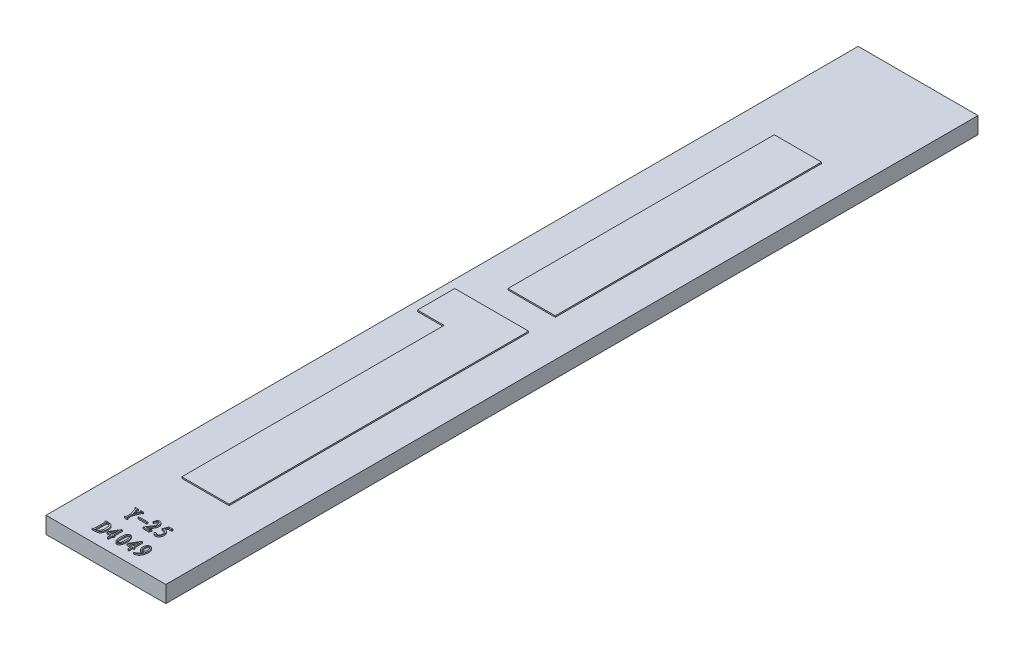
from build123d import *

# Parameters (mm, degrees)
SKETCH1_W           = 9
SKETCH1_H           = 61
BOSS_EXTRUDE1_DEPTH = 1.25
SKETCH2_W           = 3.55
SKETCH2_H           = 20
BOSS_EXTRUDE2_DEPTH = 0.1
SKETCH4_W           = 0.666666667
SKETCH4_H           = 0.083333333
BOSS_EXTRUDE3_DEPTH = 0.1
BOSS_EXTRUDE4_DEPTH = 0.1


with BuildPart() as part:
    # Sketch1 → Boss-Extrude1 (new body)
    with BuildSketch(Plane(origin=(0, 0, 0), x_dir=(1, 0, 0), z_dir=(0, 1, 0))):
        with Locations((4.5, 30.5)):
            Rectangle(SKETCH1_W, SKETCH1_H)
    extrude(amount=BOSS_EXTRUDE1_DEPTH)

    # Sketch2 → Boss-Extrude2 (add)
    with BuildSketch(Plane(origin=(0, 1.25, 0), x_dir=(1, 0, 0), z_dir=(0, 1, 0))):
        Polygon((2.7, 7.5), (6.25, 7.5), (6.25, 30), (0.7, 30), (0.7, 27.2), (2.7, 27.2), align=None)
        with Locations((4.475, 42)):
            Rectangle(SKETCH2_W, SKETCH2_H)
    extrude(amount=BOSS_EXTRUDE2_DEPTH)

    # Sketch4 → Boss-Extrude3 (add)
    with BuildSketch(Plane(origin=(0, 1.25, 0), x_dir=(1, 0, 0), z_dir=(0, 1, 0))):
        with BuildLine():
            add(Edge.make_bspline(
                [(3.112430638, 2.801603821), (3.117581172, 2.801718451), (3.127409954, 2.801937201), (3.141398685, 2.803908272), (3.153687941, 2.807150558), (3.164467449, 2.811513751), (3.173308112, 2.817610015), (3.180890686, 2.824709906), (3.186470888, 2.833463912), (3.188691334, 2.839981993), (3.18981159, 2.843270488)],
                knots=[0, 0, 0, 0, 1.302072691, 2.484749895, 3.562139971, 4.511379366, 5.408236895, 6.262493732, 7.123395447, 8, 8, 8, 8], degree=3))
            Line((3.18981159, 2.843270488), (3.18981159, 3.188508583))
            Line((3.18981159, 3.188508583), (3.041002066, 3.652794297))
            add(Edge.make_bspline(
                [(3.041002066, 3.652794297), (3.038871047, 3.658879382), (3.034760977, 3.670615605), (3.026438221, 3.686643453), (3.016164612, 3.700185527), (3.004024748, 3.711065386), (2.990457739, 3.719976466), (2.974917219, 3.725734702), (2.957946602, 3.729752217), (2.946010572, 3.730030647), (2.93981159, 3.730175249)],
                knots=[0, 0, 0, 0, 1.120090753, 2.160304349, 3.126304926, 4.057980278, 4.983061327, 5.929772381, 6.924826447, 8, 8, 8, 8], degree=3))
            Line((2.93981159, 3.730175249), (2.93981159, 3.765889535))
            Line((2.93981159, 3.765889535), (3.18981159, 3.765889535))
            Line((3.18981159, 3.765889535), (3.18981159, 3.730175249))
            add(Edge.make_bspline(
                [(3.18981159, 3.730175249), (3.185235193, 3.729984155), (3.176767714, 3.729630583), (3.165196849, 3.726598153), (3.155932393, 3.721482658), (3.149071491, 3.71401788), (3.14520736, 3.704272832), (3.143441674, 3.692750595), (3.144607976, 3.679220776), (3.146899509, 3.669812381), (3.148144923, 3.664699059)],
                knots=[0, 0, 0, 0, 1.148008426, 2.124103102, 2.975698962, 3.77274816, 4.616104197, 5.568887894, 6.67872674, 8, 8, 8, 8], degree=3))
            Line((3.148144923, 3.664699059), (3.261240161, 3.265889535))
            Line((3.261240161, 3.265889535), (3.416002066, 3.664699059))
            add(Edge.make_bspline(
                [(3.416002066, 3.664699059), (3.417241452, 3.669807437), (3.419522538, 3.679209394), (3.419720463, 3.692904094), (3.416629771, 3.70462606), (3.410469082, 3.714374984), (3.401020003, 3.721691407), (3.388689171, 3.726643043), (3.3735186, 3.729617596), (3.362445838, 3.729979958), (3.356478257, 3.730175249)],
                knots=[0, 0, 0, 0, 1.154411579, 2.124691882, 2.979940139, 3.787374271, 4.615750981, 5.564913494, 6.687628387, 8, 8, 8, 8], degree=3))
            Line((3.356478257, 3.730175249), (3.356478257, 3.765889535))
            Line((3.356478257, 3.765889535), (3.570763971, 3.765889535))
            Line((3.570763971, 3.765889535), (3.570763971, 3.730175249))
            add(Edge.make_bspline(
                [(3.570763971, 3.730175249), (3.565097471, 3.730076594), (3.554231253, 3.729887411), (3.538765239, 3.727687608), (3.524922451, 3.724040734), (3.512874507, 3.71863394), (3.502273069, 3.712087558), (3.493551288, 3.703683739), (3.486264134, 3.693911629), (3.483092248, 3.68638571), (3.481478257, 3.682556202)],
                knots=[0, 0, 0, 0, 1.254413916, 2.405494607, 3.452028913, 4.413990841, 5.321667416, 6.196791605, 7.082450772, 8, 8, 8, 8], degree=3))
            Line((3.481478257, 3.682556202), (3.279097304, 3.188508583))
            Line((3.279097304, 3.188508583), (3.279097304, 2.849222868))
            add(Edge.make_bspline(
                [(3.279097304, 2.849222868), (3.280249643, 2.845399393), (3.282472632, 2.838023482), (3.288614447, 2.828300632), (3.296038715, 2.819575939), (3.306095356, 2.813201128), (3.317462547, 2.807606634), (3.330936829, 2.804466218), (3.346008769, 2.801758023), (3.356756025, 2.801657106), (3.362430638, 2.801603821)],
                knots=[0, 0, 0, 0, 0.914764513, 1.764682586, 2.627130839, 3.527870916, 4.481226645, 5.531530322, 6.696633754, 8, 8, 8, 8], degree=3))
            Line((3.362430638, 2.801603821), (3.362430638, 2.765889535))
            Line((3.362430638, 2.765889535), (3.112430638, 2.765889535))
            Line((3.112430638, 2.765889535), (3.112430638, 2.801603821))
        make_face()
        with Locations((4.023144924, 3.248032392)):
            Rectangle(SKETCH4_W, SKETCH4_H)
        with BuildLine():
            Line((4.654097304, 2.86112763), (4.886240161, 2.86112763))
            add(Edge.make_bspline(
                [(4.886240161, 2.86112763), (4.89120182, 2.86232734), (4.90117029, 2.864737676), (4.915560668, 2.870641239), (4.929700036, 2.878182253), (4.943174184, 2.887916069), (4.956389045, 2.899410907), (4.969325445, 2.912511555), (4.981761976, 2.927712183), (4.989418066, 2.938746492), (4.993383019, 2.944460964)],
                knots=[0, 0, 0, 0, 0.878382117, 1.764757949, 2.67116336, 3.633749211, 4.621162033, 5.686586957, 6.801924741, 8, 8, 8, 8], degree=3))
            Line((4.993383019, 2.944460964), (5.029097304, 2.944460964))
            Line((5.029097304, 2.944460964), (4.969573495, 2.765889535))
            Line((4.969573495, 2.765889535), (4.523144923, 2.765889535))
            Line((4.523144923, 2.765889535), (4.523144923, 2.801603821))
            add(Edge.make_bspline(
                [(4.523144923, 2.801603821), (4.533276428, 2.815720099), (4.55307626, 2.843307307), (4.582191934, 2.883534346), (4.609687964, 2.921982472), (4.635203081, 2.958826199), (4.659995164, 2.993331759), (4.682457882, 3.026525689), (4.703962794, 3.057427651), (4.723540269, 3.086730851), (4.741958777, 3.113892248), (4.758339318, 3.139589289), (4.773698078, 3.163111499), (4.787252557, 3.184935829), (4.799551189, 3.204707669), (4.809768296, 3.222884641), (4.818954916, 3.238931677), (4.833272238, 3.266385123), (4.850738573, 3.306191809), (4.867619022, 3.359471501), (4.878179555, 3.412423136), (4.881036118, 3.464353914), (4.879376769, 3.513489546), (4.873684879, 3.558578481), (4.864697368, 3.598895473), (4.853764424, 3.629098408), (4.842943811, 3.650303598), (4.83309138, 3.663744769), (4.821745626, 3.675055001), (4.80906807, 3.684545272), (4.794681549, 3.691604059), (4.778861246, 3.696685782), (4.761580121, 3.699702913), (4.743316465, 3.700720903), (4.724975364, 3.699932686), (4.707450291, 3.697051569), (4.691225574, 3.692436175), (4.676254184, 3.686043249), (4.662629825, 3.677584194), (4.650483442, 3.667013355), (4.639321173, 3.654944269), (4.626791499, 3.635935642), (4.613390541, 3.610003395), (4.599782154, 3.576770948), (4.589437113, 3.541196018), (4.584949623, 3.516524665), (4.582668733, 3.503984773)],
                knots=[0, 0, 0, 0, 1.69631524, 3.315080701, 4.847930107, 6.310785452, 7.69019844, 8.995595461, 10.223400104, 11.365530615, 12.436016475, 13.427008482, 14.340408662, 15.178432467, 15.935125256, 16.613185454, 17.213845292, 17.740106165, 19.635490543, 21.448390511, 23.187434146, 24.891106341, 26.513476491, 27.981722556, 29.321731269, 30.538418994, 31.106445655, 31.640232205, 32.157665963, 32.665613008, 33.178952369, 33.714375566, 34.282900357, 34.88659439, 35.497070761, 36.071449824, 36.616400871, 37.140161911, 37.655752223, 38.174775033, 38.708031004, 39.255244051, 40.391297374, 41.552997966, 42.756244035, 44, 44, 44, 44], degree=3))
            Line((4.582668733, 3.503984773), (4.546954447, 3.503984773))
            add(Edge.make_bspline(
                [(4.546954447, 3.503984773), (4.548447235, 3.517302462), (4.551300798, 3.542760099), (4.557339962, 3.579000045), (4.56404142, 3.611619097), (4.571712465, 3.640641723), (4.580246877, 3.66608972), (4.589560754, 3.688066149), (4.600036933, 3.706396295), (4.61535225, 3.725273796), (4.635882965, 3.743774302), (4.661279663, 3.76208135), (4.68838557, 3.774330269), (4.716372054, 3.781352569), (4.744491904, 3.784117904), (4.772334047, 3.785855753), (4.799755235, 3.784190721), (4.822382831, 3.781726559), (4.840496661, 3.777921838), (4.853888586, 3.772428175), (4.867323438, 3.765252243), (4.880767208, 3.756167143), (4.894225861, 3.745052633), (4.907614233, 3.732053567), (4.920946192, 3.717040435), (4.934253689, 3.700336944), (4.946982488, 3.681691422), (4.957644837, 3.66079171), (4.966993301, 3.638269936), (4.97441095, 3.613800999), (4.980392081, 3.58751437), (4.98451604, 3.559280674), (4.986808626, 3.529232083), (4.987805221, 3.497662748), (4.986555747, 3.464929179), (4.982450655, 3.431573766), (4.976115453, 3.397807784), (4.966974891, 3.363619089), (4.955064583, 3.329192403), (4.940503965, 3.29439891), (4.923930706, 3.259042026), (4.903862761, 3.223445528), (4.881547087, 3.186248104), (4.856694052, 3.146974312), (4.829185585, 3.10526936), (4.799591103, 3.060883918), (4.766827012, 3.014428311), (4.731462609, 2.965530295), (4.693935471, 2.913905961), (4.667600681, 2.879017151), (4.654097304, 2.86112763)],
                knots=[0, 0, 0, 0, 1.250310692, 2.390051031, 3.426959399, 4.356778373, 5.189484751, 5.929631335, 6.581185539, 7.151993547, 8.190374716, 9.151012377, 10.062443573, 10.947251191, 11.830995274, 12.695997373, 13.547300594, 14.390193962, 14.819366142, 15.268874171, 15.735172317, 16.239174092, 16.780034109, 17.361978296, 17.978718407, 18.652343773, 19.354140052, 20.08104892, 20.837471312, 21.626987473, 22.463749812, 23.351104713, 24.286746534, 25.274582321, 26.297151914, 27.339939007, 28.40778998, 29.500603315, 30.639105254, 31.804326119, 33.018982859, 34.280469881, 35.615254974, 37.066839227, 38.616913391, 40.277264392, 42.044606227, 43.921109359, 45.908515667, 48, 48, 48, 48], degree=3))
        make_face()
        with BuildLine():
            add(Edge.make_bspline(
                [(5.701716352, 3.075413345), (5.701486986, 3.085642364), (5.701036134, 3.105749033), (5.696742862, 3.13523725), (5.689651408, 3.163356716), (5.679957419, 3.190233341), (5.667316498, 3.215755997), (5.651673853, 3.239854551), (5.633634006, 3.262913658), (5.612557201, 3.284340213), (5.588580744, 3.304151292), (5.561384932, 3.321788448), (5.530874395, 3.337012951), (5.497255551, 3.34994495), (5.460520739, 3.36068329), (5.420745897, 3.369271613), (5.377777295, 3.375357704), (5.348043177, 3.377748552), (5.332668733, 3.378984773)],
                knots=[0, 0, 0, 0, 0.917758673, 1.803991995, 2.667923906, 3.517226481, 4.363886405, 5.218398847, 6.092022264, 6.987632944, 7.910780789, 8.878660533, 9.890520551, 10.966063617, 12.107781048, 13.322690178, 14.615659297, 16, 16, 16, 16], degree=3))
            Line((5.332668733, 3.378984773), (5.487430638, 3.765889535))
            Line((5.487430638, 3.765889535), (5.785049685, 3.765889535))
            Line((5.785049685, 3.765889535), (5.743383019, 3.67065144))
            Line((5.743383019, 3.67065144), (5.499335399, 3.67065144))
            Line((5.499335399, 3.67065144), (5.421954447, 3.474222868))
            add(Edge.make_bspline(
                [(5.421954447, 3.474222868), (5.43543744, 3.4716654), (5.461759706, 3.466672563), (5.499713892, 3.45665811), (5.535158843, 3.44519123), (5.568293007, 3.432638487), (5.598509706, 3.417586893), (5.626610132, 3.401687165), (5.65216044, 3.384009142), (5.675058682, 3.364442925), (5.695678968, 3.34295099), (5.713348894, 3.318771687), (5.728278946, 3.291962691), (5.740300071, 3.262537324), (5.749783179, 3.23055874), (5.756614191, 3.196026166), (5.760422137, 3.158838789), (5.761664612, 3.119872591), (5.760405692, 3.080613578), (5.756540175, 3.04248845), (5.749730248, 3.00635462), (5.740207208, 2.972132075), (5.728099765, 2.939861114), (5.713317374, 2.909441514), (5.695589482, 2.881112397), (5.675333627, 2.855114525), (5.653707148, 2.831470576), (5.631118096, 2.810521813), (5.607717977, 2.792701367), (5.583858742, 2.777489241), (5.559239852, 2.765473359), (5.533912363, 2.756627208), (5.50796705, 2.750602231), (5.481844605, 2.747663712), (5.456572353, 2.747108423), (5.433109887, 2.746893086), (5.411849266, 2.748058321), (5.392831828, 2.749903305), (5.375992566, 2.752919751), (5.361440855, 2.757055092), (5.348984611, 2.762079917), (5.335834668, 2.77014126), (5.323067621, 2.781853056), (5.31148258, 2.797201293), (5.304299812, 2.813847059), (5.302347152, 2.831115572), (5.303741859, 2.847567865), (5.309751869, 2.86205242), (5.31929329, 2.874098869), (5.332602466, 2.882409886), (5.34718887, 2.887872427), (5.362403718, 2.890980111), (5.377603387, 2.889498356), (5.392882429, 2.885541508), (5.407769225, 2.876192595), (5.420403414, 2.860443262), (5.431421013, 2.839088668), (5.436837211, 2.822576479), (5.43981159, 2.813508583)],
                knots=[0, 0, 0, 0, 1.545808417, 3.017815207, 4.418618593, 5.742433702, 7.0051059, 8.217933456, 9.377803328, 10.499454895, 11.606341578, 12.725790828, 13.863703459, 15.05531972, 16.299589297, 17.616447294, 19.01536536, 20.506504195, 22.005917965, 23.437769934, 24.819653994, 26.143469103, 27.435204746, 28.697876944, 29.947616226, 31.192987171, 32.406012533, 33.554448986, 34.658979797, 35.715647213, 36.737654915, 37.737934401, 38.732095913, 39.732375399, 40.693368948, 41.57927611, 42.375186034, 43.091112019, 43.730941629, 44.299581586, 44.793167942, 45.239032996, 46.030451586, 46.729273299, 47.393545671, 48.044632898, 48.66911846, 49.233401885, 49.786829744, 50.372396319, 50.975153468, 51.538707531, 52.103233868, 52.679834753, 53.304704394, 54.044690326, 54.926214758, 56, 56, 56, 56], degree=3))
            add(Edge.make_bspline(
                [(5.43981159, 2.813508583), (5.452162474, 2.813730705), (5.475876657, 2.81415719), (5.509958499, 2.817086894), (5.540846431, 2.822590547), (5.568625154, 2.83002199), (5.593348612, 2.839418352), (5.614965526, 2.851061509), (5.633396893, 2.865093814), (5.648569184, 2.881530779), (5.661154426, 2.899888817), (5.671895492, 2.919845687), (5.681329596, 2.941387369), (5.688659521, 2.964862791), (5.694671528, 2.990039069), (5.698768945, 3.016953386), (5.701196569, 3.045606431), (5.701539422, 3.065267281), (5.701716352, 3.075413345)],
                knots=[0, 0, 0, 0, 1.375740717, 2.641476338, 3.805546928, 4.86588406, 5.840245249, 6.745008832, 7.591426724, 8.40803176, 9.225456845, 10.064241315, 10.929448168, 11.840631474, 12.799571018, 13.81021633, 14.869953018, 16, 16, 16, 16], degree=3))
        make_face()
    extrude(amount=BOSS_EXTRUDE3_DEPTH)

    # Sketch6 → Boss-Extrude4 (add)
    # profile 1 of 5: a face of its own
    with BuildSketch(Plane(origin=(0, 1.25, 0), x_dir=(1, 0, 0), z_dir=(0, 1, 0))):
        with BuildLine():
            add(Edge.make_bspline(
                [(4.739090128, 1.653953152), (4.74464243, 1.642572568), (4.756080648, 1.619127585), (4.770090567, 1.581179998), (4.78173022, 1.539900287), (4.792129577, 1.495458742), (4.799462129, 1.447517107), (4.805590908, 1.396286512), (4.809112201, 1.341684335), (4.810898493, 1.284845406), (4.81045001, 1.227851981), (4.807984239, 1.172740122), (4.802820651, 1.120595486), (4.79583916, 1.071352755), (4.785694739, 1.025207725), (4.774035272, 0.981871076), (4.759669722, 0.941540599), (4.743002768, 0.904504254), (4.724779757, 0.87097452), (4.704543999, 0.84189206), (4.68329615, 0.816917232), (4.66035724, 0.796602988), (4.636132366, 0.780517889), (4.610151148, 0.769502524), (4.582891587, 0.76239714), (4.554637982, 0.760433152), (4.526466096, 0.762410127), (4.499520979, 0.769409596), (4.474056632, 0.780613047), (4.450346131, 0.796493115), (4.428273135, 0.816931528), (4.408103659, 0.84189232), (4.389229563, 0.871061402), (4.37230918, 0.90455865), (4.356981203, 0.941628627), (4.343804115, 0.981976788), (4.332651247, 1.025214813), (4.323343113, 1.071416812), (4.316451231, 1.120604874), (4.311388021, 1.172754414), (4.30839382, 1.227842539), (4.307273485, 1.284832076), (4.308390658, 1.341674761), (4.311369639, 1.396250759), (4.31642398, 1.447521946), (4.323295771, 1.495397308), (4.332621016, 1.539913354), (4.343741557, 1.581111797), (4.356853888, 1.619088649), (4.372384042, 1.653289996), (4.388671741, 1.68395939), (4.404766472, 1.711192807), (4.420448299, 1.73484588), (4.436199733, 1.754716472), (4.451672302, 1.770895068), (4.467111883, 1.783348183), (4.482350471, 1.792335746), (4.502597497, 1.798509563), (4.527483962, 1.80145812), (4.556772324, 1.803406045), (4.585692197, 1.801481322), (4.609794539, 1.798536637), (4.62928061, 1.792270512), (4.644037918, 1.783268711), (4.659244462, 1.770901183), (4.674463223, 1.754575766), (4.69048871, 1.734888233), (4.706319027, 1.711133372), (4.722967082, 1.683975146), (4.733533603, 1.664299707), (4.739090128, 1.653953152)],
                knots=[0, 0, 0, 0, 1.017482002, 2.096100383, 3.245942481, 4.464050679, 5.762547996, 7.14234081, 8.61084165, 10.159330965, 11.713051354, 13.191629558, 14.592407491, 15.924128784, 17.187093352, 18.388106522, 19.529785616, 20.624461962, 21.650397864, 22.59267832, 23.467967375, 24.27990102, 25.04837719, 25.794596655, 26.538216003, 27.302571261, 28.061036816, 28.798932034, 29.528910178, 30.287513756, 31.081892824, 31.938135587, 32.860653577, 33.869922099, 34.950544627, 36.082630963, 37.279058791, 38.538412174, 39.86928151, 41.270059442, 42.749251193, 44.303207409, 45.851257185, 47.318652545, 48.695913765, 49.991707208, 51.204762542, 52.349814403, 53.420378675, 54.430476733, 55.365954973, 56.210914966, 56.97280072, 57.645375484, 58.246956243, 58.768225076, 59.23644892, 59.658660367, 60.459035494, 61.245821967, 62.014910966, 62.786084466, 63.191470614, 63.649445639, 64.166108078, 64.763585019, 65.439859612, 66.205059072, 67.056109835, 68, 68, 68, 68], degree=3))
        make_face()
        with BuildLine():
            add(Edge.make_bspline(
                [(4.447423462, 0.942533399), (4.45015124, 0.934280177), (4.455324763, 0.918627062), (4.463668268, 0.896733556), (4.472177652, 0.877563103), (4.481242535, 0.86140356), (4.48998097, 0.847586904), (4.499205212, 0.836702417), (4.508672128, 0.8284822), (4.521488613, 0.821796026), (4.537649907, 0.817518961), (4.55676736, 0.815586199), (4.575559593, 0.817448286), (4.590941859, 0.82187829), (4.603106258, 0.828444609), (4.611917226, 0.836881525), (4.620921613, 0.84763415), (4.6296653, 0.861398519), (4.638706078, 0.877603979), (4.64739944, 0.896805283), (4.656502201, 0.918565119), (4.665349639, 0.943480053), (4.673843754, 0.971803888), (4.681019157, 1.004228942), (4.687069994, 1.040812178), (4.692145926, 1.081552026), (4.695674703, 1.126505968), (4.698677318, 1.175523003), (4.699962893, 1.228828077), (4.700794856, 1.284979002), (4.699958194, 1.341350341), (4.698669013, 1.395315946), (4.695644825, 1.445506692), (4.692129825, 1.492074816), (4.687033741, 1.534866975), (4.680908997, 1.573999931), (4.673787359, 1.609430638), (4.665373874, 1.641150116), (4.656167403, 1.669227855), (4.645252263, 1.693458648), (4.633521115, 1.714237559), (4.620231093, 1.731197543), (4.605774493, 1.744659839), (4.589792593, 1.75404882), (4.572655432, 1.760128449), (4.554635709, 1.761595054), (4.53663999, 1.760087108), (4.519639459, 1.754160466), (4.503996798, 1.74455698), (4.489767344, 1.73125626), (4.476960428, 1.714184779), (4.465615058, 1.693483604), (4.455433203, 1.6691759), (4.446863001, 1.641125882), (4.439127606, 1.609403429), (4.432646755, 1.573982974), (4.427238837, 1.534837763), (4.422573592, 1.492057458), (4.419193888, 1.445505575), (4.416510621, 1.395308072), (4.415008597, 1.341352597), (4.414686135, 1.284979036), (4.415004624, 1.228825746), (4.416502474, 1.175531133), (4.419165693, 1.126507154), (4.42256019, 1.081571018), (4.427198612, 1.040841585), (4.432571317, 1.004258772), (4.438997654, 0.971812365), (4.444725668, 0.951908002), (4.447423462, 0.942533399)],
                knots=[0, 0, 0, 0, 0.837318371, 1.588063525, 2.256595512, 2.855528614, 3.371956206, 3.828855314, 4.22588514, 4.571123252, 5.211979743, 5.823459694, 6.413795224, 7.020708911, 7.35352855, 7.734517243, 8.186840906, 8.703268497, 9.302201599, 9.973688479, 10.732303747, 11.574278234, 12.519566182, 13.57927191, 14.771097569, 16.090919092, 17.53312208, 19.114568118, 20.821487341, 22.669402391, 24.524396641, 26.252546021, 27.869331708, 29.367981921, 30.751055998, 32.01973937, 33.183262711, 34.230790244, 35.180046561, 36.02611856, 36.787470794, 37.472993127, 38.094473346, 38.678492207, 39.247161774, 39.830450691, 40.406693806, 40.975363373, 41.547240947, 42.16349736, 42.840337187, 43.594678906, 44.432266602, 45.374926275, 46.417201326, 47.576646698, 48.842185377, 50.223664003, 51.72176228, 53.33816041, 55.06630979, 56.92123649, 58.76908373, 60.476002953, 62.057052771, 63.498682212, 64.816831727, 66.005309347, 67.060535974, 68, 68, 68, 68], degree=3))
        make_face(mode=Mode.SUBTRACT)
    # profile 2 of 5: a face of its own
    with BuildSketch(Plane(origin=(0, 1.25, 0), x_dir=(1, 0, 0), z_dir=(0, 1, 0))):
        with BuildLine():
            add(Edge.make_bspline(
                [(2.682652738, 0.820619819), (2.687814996, 0.820747188), (2.697713443, 0.820991413), (2.711724891, 0.82399898), (2.72428452, 0.828396042), (2.734795525, 0.835311895), (2.744011538, 0.843602336), (2.751205571, 0.854143168), (2.7568441, 0.866448456), (2.758943551, 0.875462889), (2.760033691, 0.880143629)],
                knots=[0, 0, 0, 0, 1.150371848, 2.20579727, 3.187074628, 4.101909412, 4.995909181, 5.938140712, 6.929380532, 8, 8, 8, 8], degree=3))
            Line((2.760033691, 0.880143629), (2.760033691, 1.707524581))
            add(Edge.make_bspline(
                [(2.760033691, 1.707524581), (2.758443004, 1.710812895), (2.755295218, 1.71732009), (2.748894973, 1.726011557), (2.740906138, 1.733141064), (2.731867695, 1.739240833), (2.721235161, 1.743533857), (2.709570085, 1.746856213), (2.69653572, 1.748866561), (2.687436631, 1.749079365), (2.682652738, 1.749191248)],
                knots=[0, 0, 0, 0, 0.935251606, 1.850754977, 2.744090757, 3.668849662, 4.631031247, 5.668626053, 6.774268272, 8, 8, 8, 8], degree=3))
            Line((2.682652738, 1.749191248), (2.682652738, 1.784905533))
            Line((2.682652738, 1.784905533), (2.926700357, 1.784905533))
            add(Edge.make_bspline(
                [(2.926700357, 1.784905533), (2.943042628, 1.783612512), (2.974770561, 1.781102158), (3.020483162, 1.773330759), (3.062951049, 1.762613783), (3.10205121, 1.748568568), (3.137818869, 1.731284485), (3.170337397, 1.711042469), (3.199161528, 1.687111848), (3.225105015, 1.660319453), (3.247463599, 1.629639503), (3.267035621, 1.595459272), (3.283127158, 1.55732135), (3.296747203, 1.515544911), (3.306801943, 1.469881778), (3.314373233, 1.420476471), (3.318542649, 1.367287276), (3.32008505, 1.311434246), (3.318518179, 1.255067595), (3.314293891, 1.200352208), (3.30675905, 1.148452838), (3.29651409, 1.099271684), (3.283026566, 1.052944399), (3.266845926, 1.00925936), (3.247168493, 0.968621529), (3.228890179, 0.936387516), (3.211298577, 0.91236602), (3.194957623, 0.895902888), (3.176155639, 0.880301651), (3.154275438, 0.866357018), (3.13006291, 0.853036488), (3.102932485, 0.841189824), (3.073152227, 0.830481879), (3.040654826, 0.820697374), (3.005318082, 0.812574418), (2.967357917, 0.804891382), (2.926551228, 0.798994262), (2.8830661, 0.793524113), (2.836794797, 0.789746909), (2.787845168, 0.786795769), (2.736158705, 0.785388905), (2.700804369, 0.785069515), (2.682652738, 0.784905533)],
                knots=[0, 0, 0, 0, 1.172240782, 2.275863581, 3.312445736, 4.301874109, 5.242329815, 6.149506285, 7.034618434, 7.915787832, 8.810541892, 9.7429559, 10.727273807, 11.766292461, 12.882167044, 14.068002195, 15.339269347, 16.696047765, 18.063336138, 19.371279044, 20.619512496, 21.812411093, 22.961989922, 24.06825131, 25.140452033, 26.189001953, 26.714691608, 27.264885542, 27.843741229, 28.459045194, 29.117732443, 29.81908992, 30.57407251, 31.380710697, 32.24521049, 33.166893033, 34.150494761, 35.193760284, 36.301756457, 37.470786713, 38.701450783, 40, 40, 40, 40], degree=3))
            Line((2.682652738, 0.784905533), (2.682652738, 0.820619819))
        make_face()
        with BuildLine():
            add(Edge.make_bspline(
                [(2.849319405, 0.862286486), (2.851627412, 0.860804796), (2.856664882, 0.857570853), (2.865942725, 0.854271526), (2.876988441, 0.851197971), (2.890096077, 0.848550352), (2.905273677, 0.846648172), (2.922496262, 0.845412016), (2.94175547, 0.844548781), (2.962659803, 0.844084889), (2.984572433, 0.84571683), (3.006218927, 0.851588376), (3.027044253, 0.861368479), (3.047293203, 0.874747263), (3.066683716, 0.892213745), (3.085442789, 0.913342633), (3.103556296, 0.938244745), (3.120724545, 0.966745709), (3.136867413, 0.998306849), (3.150574754, 1.032851934), (3.16261424, 1.069684314), (3.171939437, 1.109176925), (3.179366873, 1.151061678), (3.184978501, 1.195418458), (3.18783428, 1.242315518), (3.188999821, 1.290857877), (3.187839755, 1.339327129), (3.184979473, 1.386077688), (3.179364864, 1.430213796), (3.171962274, 1.471810186), (3.162649737, 1.510872562), (3.150572677, 1.547107449), (3.136872747, 1.581001236), (3.120709809, 1.611886046), (3.10359436, 1.639826644), (3.085143898, 1.664005497), (3.066251448, 1.684700622), (3.046518125, 1.701747816), (3.02588303, 1.714944178), (3.004379856, 1.7243384), (2.982158306, 1.730326016), (2.959625621, 1.731731253), (2.938222442, 1.73076759), (2.918584826, 1.7295628), (2.901306197, 1.726537621), (2.886198552, 1.723060834), (2.87347259, 1.71800124), (2.863102108, 1.711776774), (2.85477273, 1.704482189), (2.851101153, 1.698515394), (2.849319405, 1.695619819)],
                knots=[0, 0, 0, 0, 0.297691673, 0.649743506, 1.065081579, 1.546691922, 2.103306008, 2.729080002, 3.425737944, 4.201693079, 5.004837427, 5.808141097, 6.62772814, 7.499631393, 8.440267153, 9.45995791, 10.570308477, 11.78714675, 13.078576136, 14.424353997, 15.82830647, 17.293105368, 18.837079117, 20.457289414, 22.156794925, 23.949042428, 25.741289931, 27.432813797, 29.045086447, 30.581186809, 32.030439673, 33.411578569, 34.7351356, 36.005207252, 37.20160281, 38.297510403, 39.31074885, 40.246918436, 41.127910914, 41.966101869, 42.792608005, 43.618998008, 44.411273649, 45.125393261, 45.757930377, 46.318610529, 46.810279472, 47.241044858, 47.631693206, 48, 48, 48, 48], degree=3))
            Line((2.849319405, 1.695619819), (2.849319405, 0.862286486))
        make_face(mode=Mode.SUBTRACT)
    # profile 3 of 5: a face of its own
    with BuildSketch(Plane(origin=(0, 1.25, 0), x_dir=(1, 0, 0), z_dir=(0, 1, 0))):
        Polygon((3.920747977, 1.808715057), (3.920747977, 1.165857914), (4.00408131, 1.165857914), (4.00408131, 1.070619819), (3.920747977, 1.070619819), (3.920747977, 0.784905533), (3.831462262, 0.784905533), (3.831462262, 1.070619819), (3.492176548, 1.070619819), (3.492176548, 1.177762676), (3.873128929, 1.808715057), align=None)
        Polygon((3.831462262, 1.165857914), (3.831462262, 1.659905533), (3.545747977, 1.165857914), align=None, mode=Mode.SUBTRACT)
    # profile 4 of 5: a face of its own
    with BuildSketch(Plane(origin=(0, 1.25, 0), x_dir=(1, 0, 0), z_dir=(0, 1, 0))):
        Polygon((5.4445575, 1.808715057), (5.4445575, 1.165857914), (5.527890834, 1.165857914), (5.527890834, 1.070619819), (5.4445575, 1.070619819), (5.4445575, 0.784905533), (5.355271786, 0.784905533), (5.355271786, 1.070619819), (5.015986072, 1.070619819), (5.015986072, 1.177762676), (5.396938453, 1.808715057), align=None)
        Polygon((5.355271786, 1.165857914), (5.355271786, 1.659905533), (5.0695575, 1.165857914), align=None, mode=Mode.SUBTRACT)
    # profile 5 of 5: a face of its own
    with BuildSketch(Plane(origin=(0, 1.25, 0), x_dir=(1, 0, 0), z_dir=(0, 1, 0))):
        with BuildLine():
            add(Edge.make_bspline(
                [(6.289795596, 1.406819114), (6.28966979, 1.393217099), (6.289419203, 1.366123954), (6.286041272, 1.325608375), (6.28135475, 1.285344217), (6.274437334, 1.245328853), (6.265684062, 1.20565262), (6.254688773, 1.166295359), (6.242323942, 1.127040221), (6.227537995, 1.08856116), (6.211396803, 1.051397173), (6.194093342, 1.016133343), (6.175017313, 0.983577219), (6.155062197, 0.95310131), (6.133267524, 0.925405124), (6.110720916, 0.899572815), (6.086323853, 0.876701752), (6.060798794, 0.856034162), (6.034079367, 0.837540232), (6.006207902, 0.820873513), (5.977017028, 0.806405438), (5.946710191, 0.793525087), (5.915166194, 0.782565837), (5.882441909, 0.773235636), (5.848491112, 0.765909444), (5.825314005, 0.762711556), (5.813605119, 0.761096009)],
                knots=[0, 0, 0, 0, 1.108234654, 2.207434812, 3.311323939, 4.411127618, 5.515455316, 6.621162561, 7.740539739, 8.868408293, 9.978825484, 11.042148927, 12.067310494, 13.052323899, 14.008324617, 14.93740104, 15.844026504, 16.729799855, 17.611982178, 18.49017086, 19.374038928, 20.265040865, 21.172318884, 22.093699957, 23.036952798, 24, 24, 24, 24], degree=3))
            Line((5.813605119, 0.761096009), (5.813605119, 0.796810295))
            add(Edge.make_bspline(
                [(5.813605119, 0.796810295), (5.824229458, 0.799454349), (5.845163316, 0.804664109), (5.875254508, 0.814878236), (5.903778233, 0.826541836), (5.930401764, 0.84018208), (5.955266048, 0.855666538), (5.978188686, 0.873031568), (5.999837601, 0.89162935), (6.025231144, 0.91938927), (6.053757866, 0.955725435), (6.083603967, 1.00115347), (6.107737987, 1.04838497), (6.123374137, 1.088763606), (6.133733935, 1.12058245), (6.141091312, 1.142726206), (6.147445272, 1.163435406), (6.153386864, 1.182448655), (6.158724805, 1.199925269), (6.163306629, 1.215739161), (6.167384808, 1.229967125), (6.169666484, 1.23897108), (6.170747977, 1.243238867)],
                knots=[0, 0, 0, 0, 1.081513969, 2.130980523, 3.137038002, 4.124365175, 5.083488386, 6.027537773, 6.964128193, 7.89919712, 9.739917956, 11.524518695, 13.262075885, 14.970665001, 15.79737628, 16.568987143, 17.276418765, 17.937931299, 18.537512503, 19.08215638, 19.564951083, 20, 20, 20, 20], degree=3))
            add(Edge.make_bspline(
                [(6.170747977, 1.243238867), (6.162177437, 1.237464981), (6.145711377, 1.226371962), (6.121487332, 1.211018422), (6.099393729, 1.196745835), (6.078714012, 1.183442933), (6.056875388, 1.172365994), (6.031333809, 1.166621123), (6.00245821, 1.164166797), (5.97629426, 1.164764866), (5.954265786, 1.168336574), (5.937654906, 1.173642908), (5.921498981, 1.181721103), (5.906204771, 1.192751962), (5.890935382, 1.205831624), (5.876472919, 1.22188287), (5.862429974, 1.240464197), (5.84885404, 1.261255406), (5.836290194, 1.284021996), (5.825612285, 1.308595561), (5.816210762, 1.334465669), (5.80889825, 1.361798914), (5.802819841, 1.390400373), (5.798693001, 1.420388498), (5.796369337, 1.451825627), (5.795403484, 1.484201504), (5.796472125, 1.516528187), (5.799526879, 1.547836299), (5.804613133, 1.577670358), (5.811502218, 1.606128623), (5.820919218, 1.632991195), (5.832131803, 1.658385874), (5.845335349, 1.68240346), (5.860847366, 1.704354834), (5.876865903, 1.724501573), (5.892873082, 1.742493165), (5.908341247, 1.758277549), (5.923941361, 1.771234005), (5.938807713, 1.782332401), (5.953800224, 1.790460875), (5.968330479, 1.79675811), (5.987750348, 1.800827349), (6.012016126, 1.803193851), (6.041488311, 1.80489258), (6.071674026, 1.803062898), (6.097318702, 1.800979511), (6.118375001, 1.796412891), (6.134138045, 1.788988454), (6.149883883, 1.77870035), (6.165623345, 1.765269283), (6.181214761, 1.748658323), (6.196587165, 1.72878399), (6.212301652, 1.706035119), (6.227701897, 1.680277015), (6.242480849, 1.652265792), (6.254962827, 1.622004958), (6.265801055, 1.590291447), (6.274610387, 1.556842186), (6.28144756, 1.521711946), (6.286128129, 1.484884392), (6.289445326, 1.446415033), (6.289677217, 1.420201077), (6.289795596, 1.406819114)],
                knots=[0, 0, 0, 0, 1.172239559, 2.252153155, 3.253427421, 4.155650977, 5.043079479, 6.013584551, 7.101927713, 8.328091548, 8.970862171, 9.627326233, 10.298395876, 11.010709522, 11.761219724, 12.575463181, 13.455815415, 14.401513458, 15.390180276, 16.401674709, 17.437977082, 18.509848742, 19.608550955, 20.753316082, 21.94063557, 23.183211102, 24.42603829, 25.607254776, 26.748889175, 27.856881905, 28.924628531, 29.97336331, 31.003308868, 32.027740415, 33.01851377, 33.921968926, 34.75902285, 35.52220466, 36.220924788, 36.858974878, 37.453438891, 38.009548111, 39.100474331, 40.218675164, 41.353532413, 42.527312367, 43.135928828, 43.785154213, 44.49040828, 45.265337599, 46.126293446, 47.070226166, 48.113113183, 49.261151845, 50.472948749, 51.702254168, 52.970296096, 54.272514721, 55.622964866, 57.027176992, 58.482403409, 60, 60, 60, 60], degree=3))
        make_face()
        with BuildLine():
            add(Edge.make_bspline(
                [(6.146938453, 1.656819114), (6.143318947, 1.665002564), (6.136382025, 1.680686464), (6.123133761, 1.701776237), (6.107567145, 1.718963312), (6.090049818, 1.732551102), (6.070511682, 1.742381231), (6.049002563, 1.748656663), (6.025506584, 1.750854998), (6.005070262, 1.750013237), (5.988414334, 1.747349563), (5.976482497, 1.743304649), (5.965341854, 1.737762156), (5.955001213, 1.730573285), (5.945569998, 1.72162734), (5.936665833, 1.711324671), (5.929009204, 1.699171026), (5.921898806, 1.68562291), (5.915531833, 1.670435426), (5.910140306, 1.653578337), (5.905140121, 1.635311488), (5.901665823, 1.615270265), (5.898133026, 1.593784879), (5.896155483, 1.57056972), (5.894572803, 1.545800907), (5.893456875, 1.511546245), (5.893802711, 1.470217888), (5.895470497, 1.424264972), (5.898438046, 1.383803911), (5.903827836, 1.349022545), (5.909997658, 1.319536391), (5.918565882, 1.295757853), (5.928372879, 1.276990079), (5.944114002, 1.260327849), (5.965744835, 1.247471112), (5.991278864, 1.236598323), (6.017202365, 1.231478464), (6.042761804, 1.233566602), (6.067031062, 1.239318715), (6.090195787, 1.246585254), (6.111917076, 1.255562837), (6.131817499, 1.266522641), (6.149685541, 1.278872969), (6.163562634, 1.294053323), (6.174152697, 1.310757658), (6.179119814, 1.32664192), (6.181979657, 1.340470506), (6.183665509, 1.352709361), (6.185189214, 1.366603228), (6.186548103, 1.382181817), (6.18732946, 1.399392305), (6.188019454, 1.418205215), (6.188398461, 1.438710715), (6.188924667, 1.468642932), (6.186735579, 1.508062001), (6.178824208, 1.556633102), (6.165825392, 1.606713244), (6.153353116, 1.639801412), (6.146938453, 1.656819114)],
                knots=[0, 0, 0, 0, 1.114549983, 2.136078201, 3.089322438, 3.990763634, 4.883834809, 5.799865472, 6.766961346, 7.812240239, 8.342352177, 8.863765972, 9.37584268, 9.8891469, 10.427115105, 10.992462633, 11.581933881, 12.21293208, 12.898549058, 13.631430838, 14.417991329, 15.25699741, 16.165162239, 17.13134664, 18.159302846, 19.259150159, 21.402681483, 23.309434019, 24.991392041, 26.455322537, 27.695318162, 28.738547998, 29.599811699, 30.312787264, 31.565473848, 32.703492183, 33.76533729, 34.820722291, 35.871924852, 36.87140624, 37.84451368, 38.795642922, 39.700799886, 40.537000923, 41.34295175, 42.145354873, 42.594490228, 43.10360883, 43.684259562, 44.336959532, 45.052402351, 45.831513221, 46.68361871, 47.608855027, 49.563094327, 51.594659523, 53.734272641, 56, 56, 56, 56], degree=3))
        make_face(mode=Mode.SUBTRACT)
    extrude(amount=BOSS_EXTRUDE4_DEPTH)


solid = part.part
